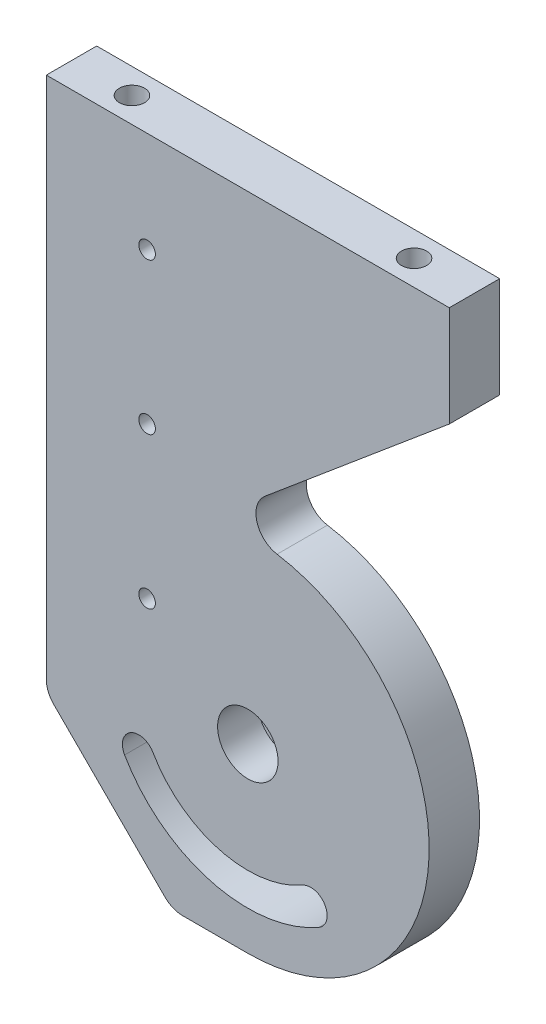
SolidWorks part; units mm, degrees
material "6061"
ref_plane "前视基准面" through (0, 0, 0) normal (0, 0, 1) x (1, 0, 0)
ref_plane "上视基准面" through (0, 0, 0) normal (0, 1, 0) x (1, 0, 0)
ref_plane "右视基准面" through (0, 0, 0) normal (1, 0, 0) x (0, 0, -1)
sketch "草图1" plane through (0, 0, 0) normal (0, 0, 1) x (1, 0, 0)
  line L1 (-40, -85) -> (40, -85)
  line L2 (-40, -85) -> (-40, 85)
  line L3 (-40, 85) -> (40, 85)
  line L4 (40, -85) -> (40, 85)
  line L5 (-40, -85) -> (40, 85) construction
  line L6 (-40, 85) -> (40, -85) construction
  point P0 (0, 0)
  dimension "D1" = 80
  dimension "D2" = 170
extrude "凸台-拉伸1" add sketch "草图1" along normal mid plane 10
hole_wizard "孔1" positions "草图5" profile "草图4" legacy end condition through all
sketch "草图5" plane through (0, 0, 5) normal (0, 0, -1) x (-1, 0, 0)
  point P0 (0, -10)
  dimension "D1" = 10
sketch "草图4" plane through (0, -10, 5) normal (1, 0, 0) x (0, -1, 0)
  line L0 (0, 0) -> (0, 10)
  line L1 (0, 10) -> (5, 10)
  line L2 (5, 10) -> (5, 8)
  line L3 (5, 8) -> (6, 8)
  line L4 (6, 8) -> (6, 0)
  line L5 (6, 0) -> (0, 0)
  line L6 (0, 110) -> (0, -10) construction
  dimension "直径" = 10
  dimension "深度" = 10
  dimension "柱坑直径" = 12
  dimension "柱坑深度" = 8
sketch "草图6" plane through (0, 0, -5) normal (0, 0, -1) x (-1, 0, 0)
  line L0 (0, -10) -> (-12.5, -31.6506) construction
  line L1 (0, -10) -> (21.6506, -22.5) construction
  line L2 (0, -10) -> (0, -48.1062) construction
  circle A0 centre (0, -10) radius 25 construction
  arc A1 (-14.125, -34.4652) -> (24.4652, -24.125) centre (0, -10) ccw
  arc A2 (-10.875, -28.8361) -> (18.8361, -20.875) centre (0, -10) ccw
  arc A3 (-10.875, -28.8361) -> (-14.125, -34.4652) centre (-12.5, -31.6506) ccw
  arc A4 (24.4652, -24.125) -> (18.8361, -20.875) centre (21.6506, -22.5) ccw
  circle A5 centre (0, -10) radius 21.75 construction
  circle A6 centre (0, -10) radius 28.25 construction
  dimension "D1" = 50
  dimension "D2" = 30
  dimension "D3" = 60
  dimension "D4" = 3.25
extrude "切除-拉伸2" cut sketch "草图6" against normal through all
sketch "草图11" plane through (0, 0, -5) normal (0, 0, -1) x (-1, 0, 0)
  line L0 (0, -46) -> (15, -46)
  line L2 (15, -46) -> (40, -21)
  line L3 (-40, 85) -> (40, 85) construction
  line L4 (7.3928, 25.2328) -> (-40, 65)
  line L5 (-40, -85) -> (-40, 85) construction
  line L6 (-40, 65) -> (-40, -85)
  line L7 (-40, -85) -> (40, -85)
  line L8 (40, -85) -> (40, -21)
  line L9 (40, 85) -> (40, -85) construction
  arc A0 (7.3928, 25.2328) -> (0, -46) centre (0, -10) ccw
  dimension "D1" = 72
  dimension "D2" = 130
  dimension "D3" = 25
  dimension "D4" = 45
  dimension "D5" = 20
extrude "切除-拉伸4" cut sketch "草图11" against normal through all
fillet "圆角1" radius 5 3 edges at (-7.3928, 25.2328, 0) (-40, -21, 0) (-15, -46, 0)
hole_wizard "M6 螺纹孔1" positions "草图15" profile "草图14" tap size "M6" standard "GB"
sketch "草图15" plane through (0, 85, 0) normal (0, 1, 0) x (1, 0, 0)
  point P0 (-28, 0)
  point P2 (28, 0)
  dimension "D1" = 56
  dimension "D2" = 28
sketch "草图14" plane through (-28, 85, 0) normal (1, 0, 0) x (0, 0, 1)
  line L0 (0, 0) -> (0, 18.5022)
  line L1 (0, 18.5022) -> (2.5, 17)
  line L2 (2.5, 17) -> (2.5, 0)
  line L5 (2.5, 0) -> (0, 0)
  line L10 (0, 18.5022) -> (-2.5, 17) construction
  line L11 (0, -6.35) -> (0, 107.95) construction
  dimension "螺纹孔钻头直径" = 5
  dimension "螺纹孔钻头深度" = 17
  dimension "导头角度" = 118
cosmetic thread "孔螺蚊线1" parameters "D1"=12, "D2"=6
cosmetic thread "孔螺蚊线2" parameters "D1"=12, "D2"=6
hole_wizard "M4 螺纹孔1" positions "草图18" profile "草图17" tap size "M4" standard "GB" end condition through all
sketch "草图18" plane through (0, 0, -5) normal (0, 0, -1) x (-1, 0, 0)
  line L0 (20, 85) -> (20, -57.6374) construction
  line L1 (-40, 85) -> (40, 85) construction
  line L3 (40, 85) -> (40, -18.9289) construction
  point P0 (20, 35)
  point P2 (20, 65)
  point P14 (20, 5)
  dimension "D1" = 20
  dimension "D2" = 50
  dimension "D3" = 30
  dimension "D4" = 80
cosmetic thread "孔螺蚊线3" parameters "D2"=4
cosmetic thread "孔螺蚊线4" parameters "D2"=4
cosmetic thread "孔螺蚊线5" parameters "D2"=4
sketch "草图17" plane through (-20, 35, -5) normal (1, 0, 0) x (0, 1, 0)
  line L0 (0, 0) -> (0, 10)
  line L1 (0, 10) -> (1.65, 10)
  line L2 (1.65, 10) -> (1.65, 0)
  line L5 (1.65, 0) -> (0, 0)
  line L11 (0, -6.35) -> (0, 107.95) construction
  dimension "通孔螺纹孔钻头直径" = 3.3
  dimension "通孔螺纹孔钻头深度" = 10
